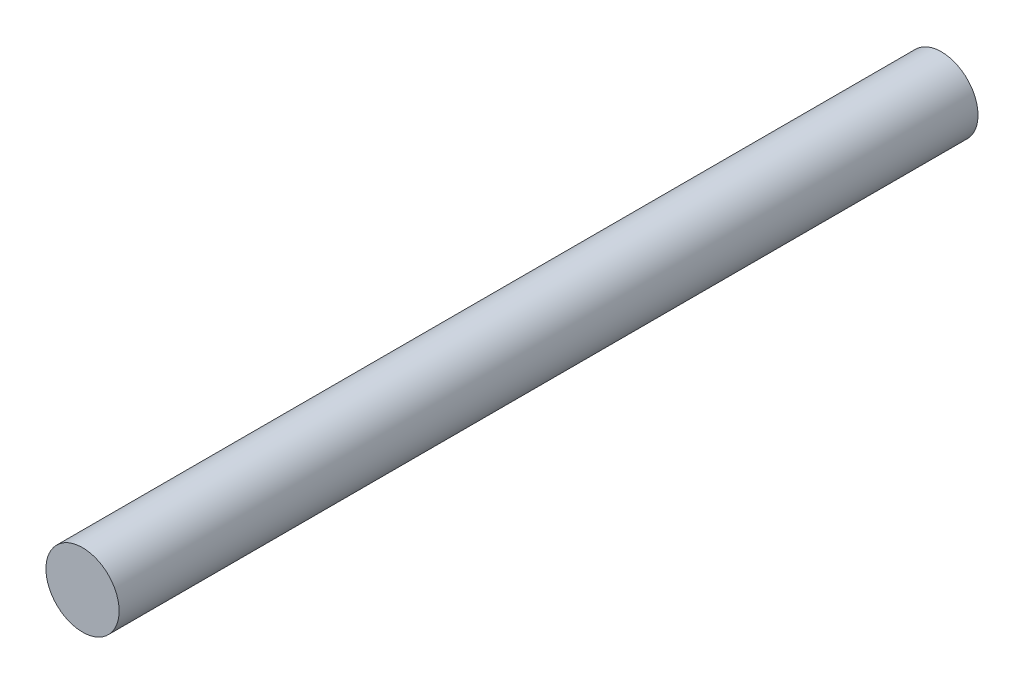
SolidWorks part; units mm, degrees
ref_plane "前视基准面" through (0, 0, 0) normal (0, 0, 1) x (1, 0, 0)
ref_plane "上视基准面" through (0, 0, 0) normal (0, 1, 0) x (1, 0, 0)
ref_plane "右视基准面" through (0, 0, 0) normal (1, 0, 0) x (0, 0, -1)
sketch "草图1" plane through (0, 0, 0) normal (0, 0, 1) x (1, 0, 0)
  circle A0 centre (0, 0) radius 15
  dimension "D1" = 30
extrude "凸台-拉伸1" add sketch "草图1" along normal blind 400
sketch "草图2" plane through (0, 0, 400) normal (0, 0, 1) x (1, 0, 0)
  circle A1 centre (0, 0) radius 15 construction
  circle A2 centre (0, 0) radius 15
extrude "切除-拉伸1" cut sketch "草图2" against normal blind 48
